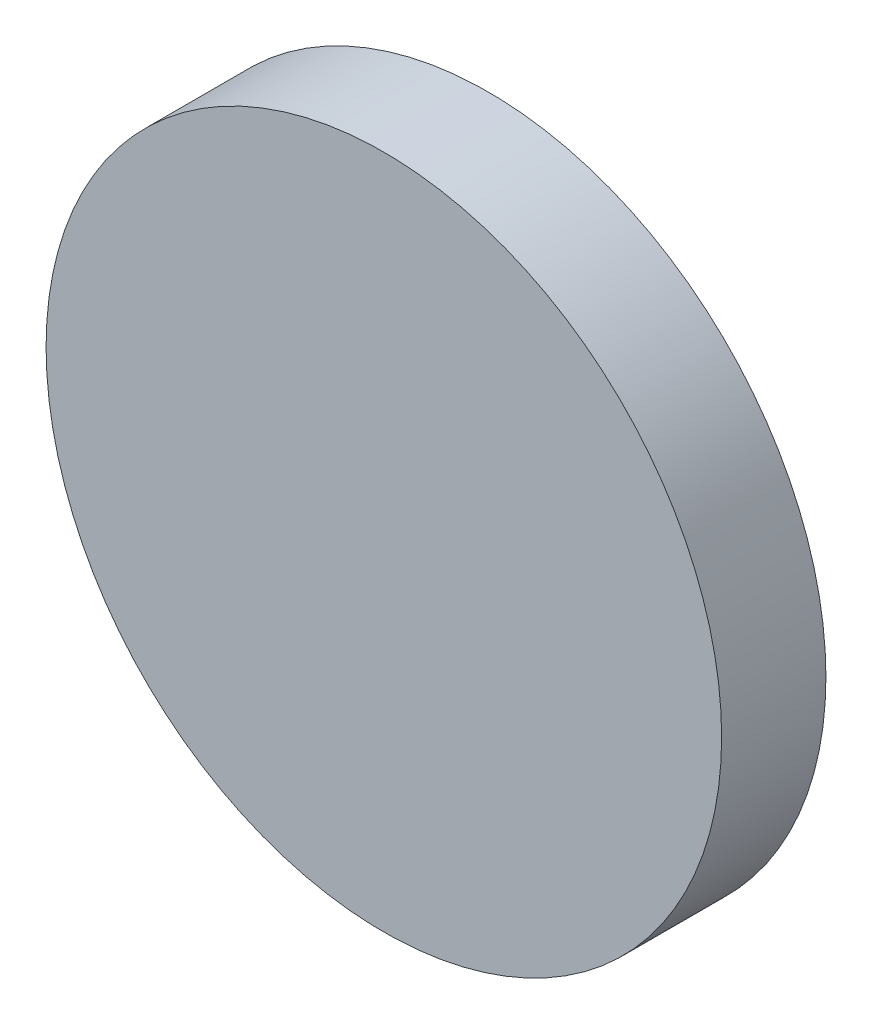
SolidWorks part; units mm, degrees
ref_plane "Front Plane" through (0, 0, 0) normal (0, 0, 1) x (1, 0, 0)
ref_plane "Top Plane" through (0, 0, 0) normal (0, 1, 0) x (1, 0, 0)
ref_plane "Right Plane" through (0, 0, 0) normal (1, 0, 0) x (0, 0, -1)
sketch "Sketch2" plane through (0, 0, 0) normal (0, 0, 1) x (1, 0, 0)
  circle A0 centre (0, 0) radius 74.5
  dimension "D1" = 149
extrude "Boss-Extrude1" add sketch "Sketch2" along normal blind 23
